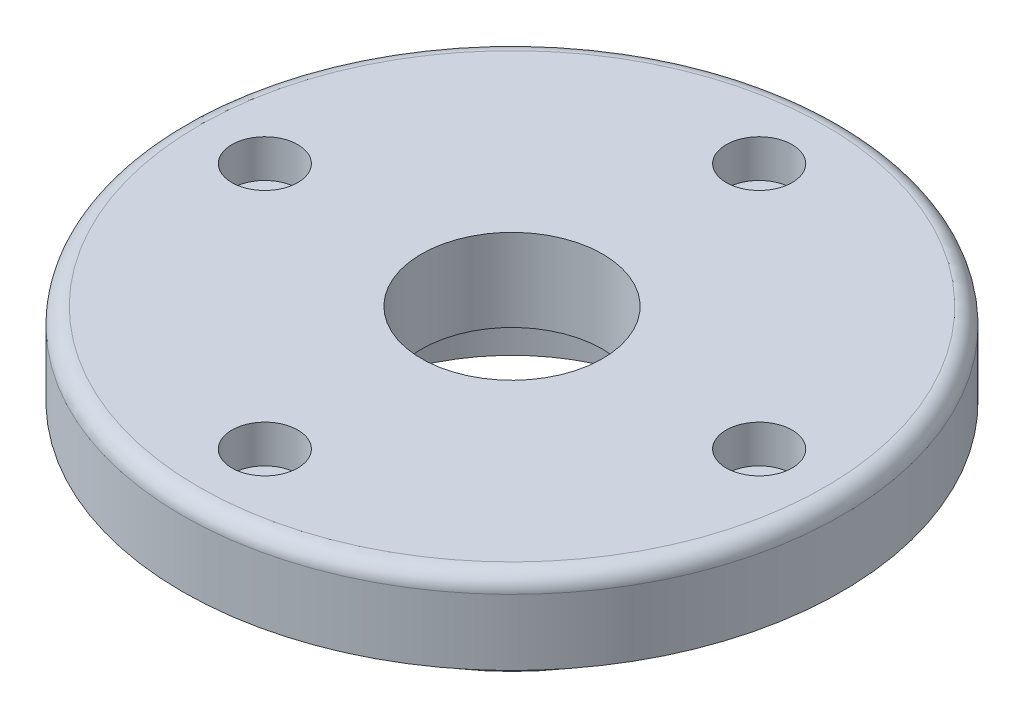
SolidWorks part; units mm, degrees
ref_plane "Front Plane" through (0, 0, 0) normal (0, 0, 1) x (1, 0, 0)
ref_plane "Top Plane" through (0, 0, 0) normal (0, 1, 0) x (1, 0, 0)
ref_plane "Right Plane" through (0, 0, 0) normal (1, 0, 0) x (0, 0, -1)
sketch "Sketch1" plane through (0, 0, 0) normal (0, 1, 0) x (1, 0, 0)
  circle A0 centre (0, 0) radius 26
  circle A1 centre (0, 0) radius 21
  dimension "D1" = 52
  dimension "D2" = 5
extrude "Boss-Extrude1" add sketch "Sketch1" along normal blind 10
sketch "Sketch2" plane through (0, 10, 0) normal (0, 1, 0) x (1, 0, 0)
  circle A0 centre (0, 0) radius 40
  dimension "D1" = 80
extrude "Boss-Extrude2" add sketch "Sketch2" along normal blind 10
sketch "Sketch3" plane through (0, 10, 0) normal (0, -1, 0) x (1, 0, 0)
  circle A0 centre (0, 0) radius 11
  dimension "D1" = 22
extrude "Cut-Extrude1" cut sketch "Sketch3" against normal blind 10
fillet "Fillet1" radius 2 1 edges at (0, 20, 40)
sketch "Sketch4" plane through (0, 20, 0) normal (0, 1, 0) x (1, 0, 0)
  circle A0 centre (0, 0) radius 30 construction
  point P3 (0, 30)
  dimension "D1" = 60
hole_wizard "Hole size (%based) hex socket head cap screw type 1" positions "Sketch5" profile "Sketch6" counterbore size "M4" standard "GB" end condition through all
sketch "Sketch5" plane through (0, 20, 0) normal (0, 1, 0) x (1, 0, 0)
  point P0 (0, 30)
sketch "Sketch6" plane through (0, 20, -30) normal (1, 0, 0) x (0, 0, 1)
  line L0 (0, 0) -> (0, 20)
  line L1 (0, 20) -> (2.25, 20)
  line L3 (2.25, 20) -> (2.25, 4.6)
  line L4 (2.25, 4.6) -> (4, 4.6)
  line L5 (4, 4.6) -> (4, 0)
  line L7 (4, 0) -> (0, 0)
  line L11 (0, -6.35) -> (0, 107.95) construction
  dimension "通孔孔直径" = 4.5
  dimension "通孔孔深度" = 20
  dimension "柱形沉头孔直径" = 8
  dimension "柱形沉头孔深度" = 4.6
pattern_circular "CirPattern1" count 4 over 360 about axis through (0, 0, 0) along (0, 1, 0) of "Hole size (%based) hex socket head cap screw type 1"
